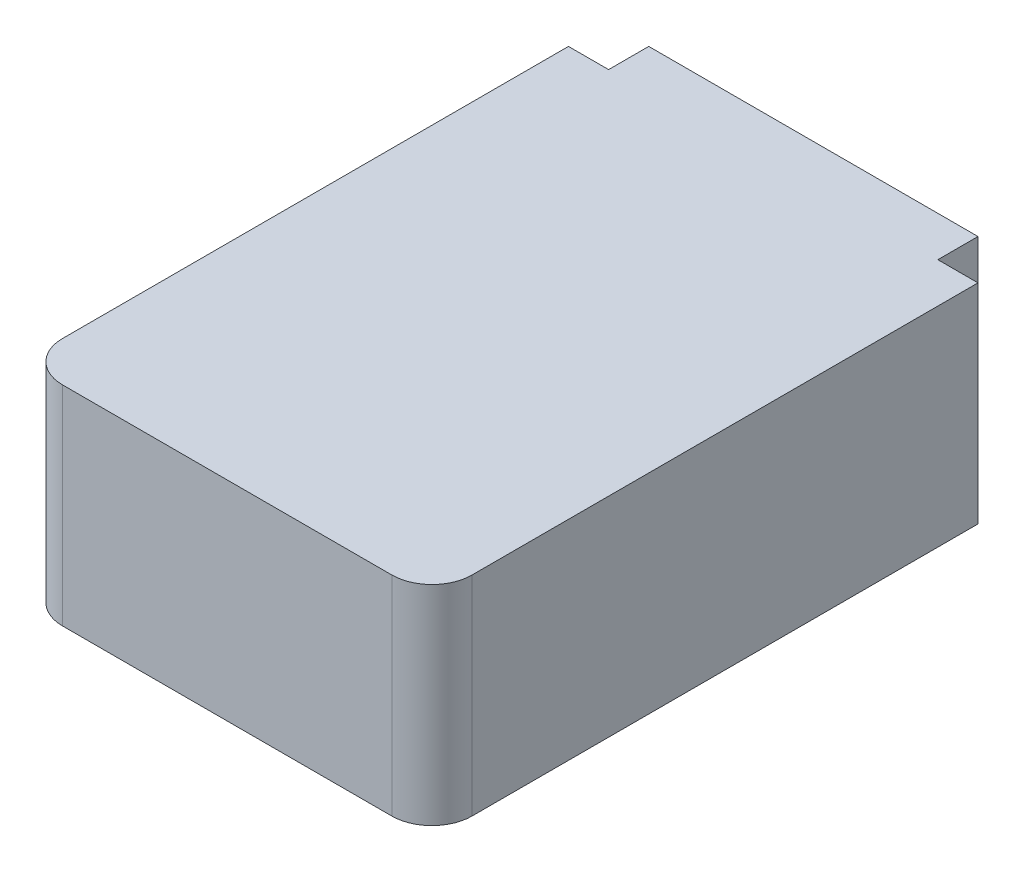
from build123d import *

# Parameters (mm, degrees)
SKETCH_1_W             = 51
SKETCH_1_H             = 73
EXTRUDE_1_DEPTH        = 26
FILLET_1_R             = 5
SKETCH_2_W             = 5
SKETCH_2_H             = 5
CUT_EXTRUDE_1_DEPTH    = 30
HOLE_WIZARD_M3_1_D     = 2.5
HOLE_WIZARD_M3_1_DEPTH = 7.5
HOLE_WIZARD_M3_1_TIP   = 0.751075774


with BuildPart() as part:
    # 草图1 → 凸台-拉伸1 (new body)
    with BuildSketch(Plane(origin=(0, 0, 0), x_dir=(1, 0, 0), z_dir=(0, 1, 0))):
        Rectangle(SKETCH_1_W, SKETCH_1_H)
    extrude(amount=EXTRUDE_1_DEPTH)

    # 圆角1
    fillet_1_edges = [part.edges().sort_by_distance(p)[0] for p in [
        (25.5, 13, 36.5),
        (-25.5, 13, 36.5),
        (-25.5, 13, -36.5),
        (25.5, 13, -36.5),
    ]]
    fillet(fillet_1_edges, radius=FILLET_1_R)

    # 草图2 → 切除-拉伸1 (cut)
    with BuildSketch(Plane.XZ):
        with Locations((23, -34)):
            Rectangle(SKETCH_2_W, SKETCH_2_H)
        with Locations((-23, -34)):
            Rectangle(SKETCH_2_W, SKETCH_2_H)
    extrude(amount=-CUT_EXTRUDE_1_DEPTH, mode=Mode.SUBTRACT)

    # M3 螺纹孔1
    with Locations(Plane(origin=(0, 0, 0), x_dir=(-1, 0, 0), z_dir=(0, -1, 0))):
        with Locations((14.8, -8.3), (-16.2, -8.3), (14.8, 21.7), (-16.2, 21.7)):
            Hole(HOLE_WIZARD_M3_1_D / 2, depth=HOLE_WIZARD_M3_1_DEPTH)
            with Locations((0, 0, -(HOLE_WIZARD_M3_1_DEPTH + HOLE_WIZARD_M3_1_TIP / 2))):  # 118° drill point
                Cone(0, HOLE_WIZARD_M3_1_D / 2, HOLE_WIZARD_M3_1_TIP, mode=Mode.SUBTRACT)


solid = part.part
